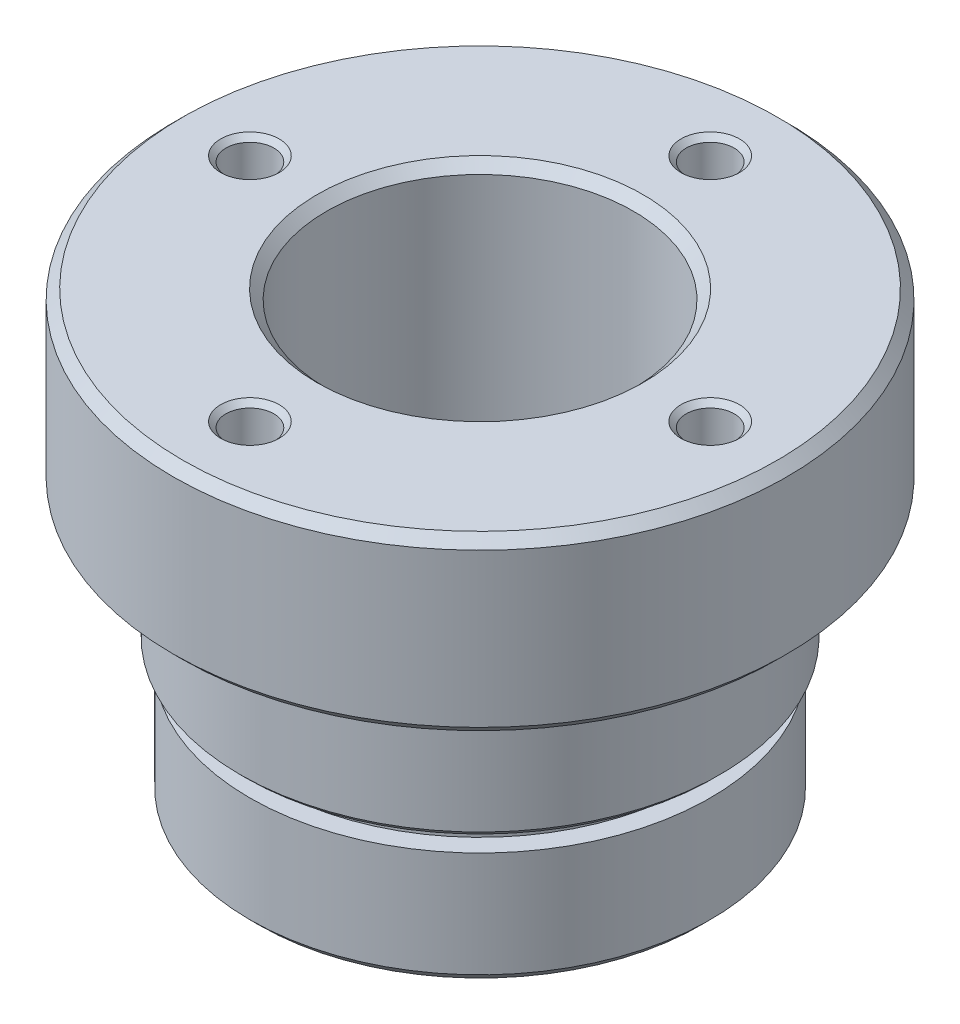
from build123d import *

# Parameters (mm, degrees)
M3_TAPPED_HOLE1_D           = 2.5
M3_TAPPED_HOLE1_DEPTH       = 7
M3_TAPPED_HOLE1_CSINK_D     = 3.05
M3_TAPPED_HOLE1_CSINK_ANGLE = 90
M3_TAPPED_HOLE1_TIP         = 0.751075774


with BuildPart() as part:
    # Sketch1 → Revolve1 (revolve)
    with BuildSketch(Plane.XY, mode=Mode.PRIVATE) as revolve1_sk:
        Polygon((8.5, 0), (15.5, 0), (16, -0.5), (16, -8.5), (15.5, -9), (12, -9), (12, -9.2), (12.5, -9.7), (12.5, -15.7), (12.2, -16), (11, -16), (11, -17), (12, -17), (12, -22.5), (11.5, -23), (8.5, -23), (8, -22.5), (8, -0.5), align=None)
    revolve(revolve1_sk.sketch.rotate(Axis((0, 0, 0), (0, -1, 0)), 90), axis=Axis((0, 0, 0), (0, -1, 0)))

    # M3 Tapped Hole1
    with Locations(Plane(origin=(0, 0, 0), x_dir=(1, 0, 0), z_dir=(0, 1, 0))):
        with Locations((-12, 0), (0, 12), (12, 0), (0, -12)):
            CounterSinkHole(M3_TAPPED_HOLE1_D / 2, M3_TAPPED_HOLE1_CSINK_D / 2, depth=M3_TAPPED_HOLE1_DEPTH, counter_sink_angle=M3_TAPPED_HOLE1_CSINK_ANGLE)
            with Locations((0, 0, -(M3_TAPPED_HOLE1_DEPTH + M3_TAPPED_HOLE1_TIP / 2))):  # 118° drill point
                Cone(0, M3_TAPPED_HOLE1_D / 2, M3_TAPPED_HOLE1_TIP, mode=Mode.SUBTRACT)


solid = part.part
